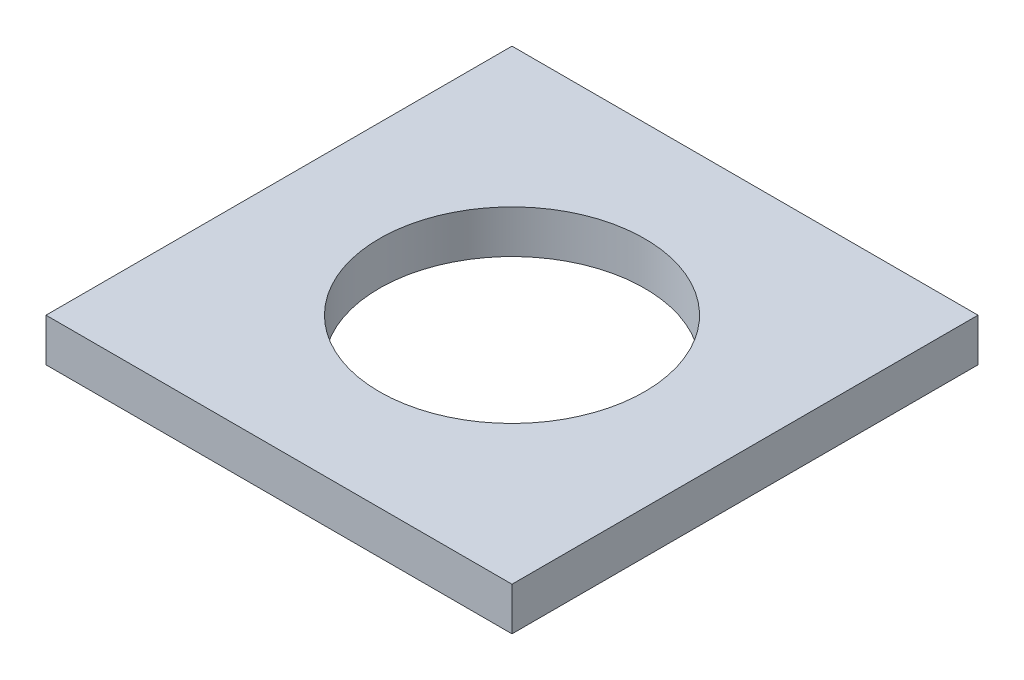
from build123d import *

# Parameters (mm, degrees)
SKETCH2_W           = 65
SKETCH2_H           = 65
SKETCH2_R           = 18.5
BOSS_EXTRUDE1_DEPTH = 3


with BuildPart() as part:
    # Sketch2 → Boss-Extrude1 (new, symmetric)
    with BuildSketch(Plane(origin=(0, 0, 0), x_dir=(1, 0, 0), z_dir=(0, 1, 0))):
        Rectangle(SKETCH2_W, SKETCH2_H)
        with Locations(Location((0, 0, 0), (0, 0, 270))):
            Circle(SKETCH2_R, mode=Mode.SUBTRACT)
    extrude(amount=BOSS_EXTRUDE1_DEPTH, both=True)


solid = part.part
